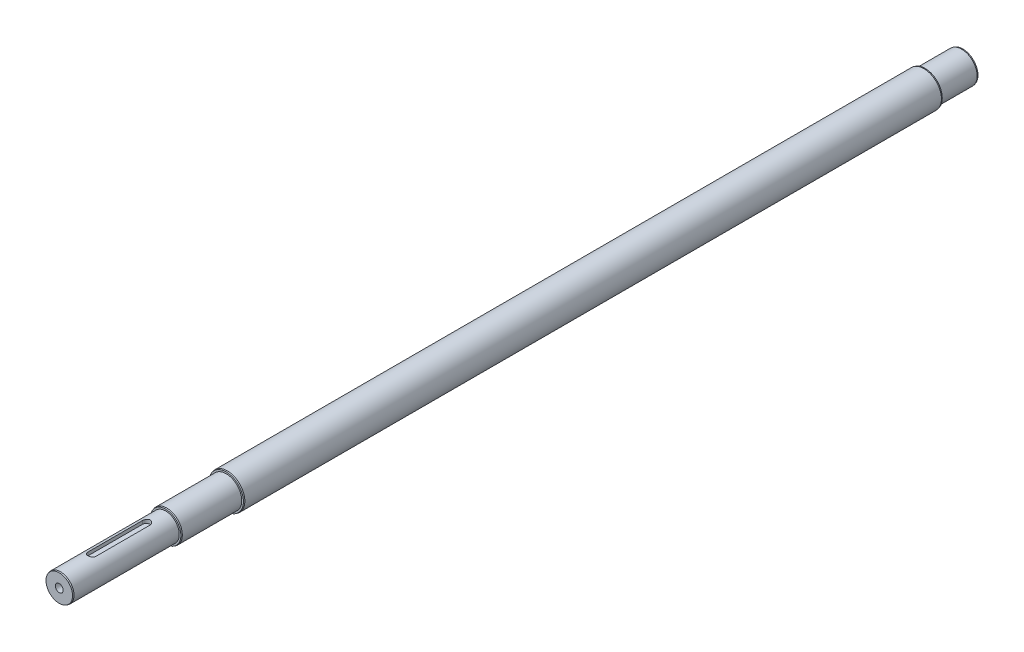
SolidWorks part; units mm, degrees
ref_plane "前视基准面" through (0, 0, 0) normal (0, 0, 1) x (1, 0, 0)
ref_plane "上视基准面" through (0, 0, 0) normal (0, 1, 0) x (1, 0, 0)
ref_plane "右视基准面" through (0, 0, 0) normal (1, 0, 0) x (0, 0, -1)
sketch "草图1" plane through (0, 0, 0) normal (0, 0, 1) x (1, 0, 0)
  circle A0 centre (0, 0) radius 22.5
  dimension "D1" = 45
extrude "凸台-拉伸1" add sketch "草图1" along normal blind 900 contours A0
sketch "草图2" plane through (0, 0, 900) normal (0, 0, 1) x (1, 0, 0)
  circle A0 centre (0, 0) radius 20
  dimension "D1" = 40
extrude "凸台-拉伸2" add sketch "草图2" along normal blind 78
sketch "草图3" plane through (0, 0, 978) normal (0, 0, 1) x (1, 0, 0)
  circle A0 centre (0, 0) radius 17.5
  dimension "D1" = 35
extrude "凸台-拉伸3" add sketch "草图3" along normal blind 137
sketch "草图4" plane through (0, 0, 0) normal (0, 0, -1) x (-1, 0, 0)
  circle A0 centre (0, 0) radius 20
  dimension "D1" = 40
extrude "凸台-拉伸4" add sketch "草图4" along normal blind 48.5
chamfer "倒角1" distance 1.5 angle 15 4 edges at (22.5, 0, 900) (-20, 0, -48.5) (17.5, 0, 1115) (20, 0, 978)
ref_plane "基准面1" through (0, 17.5, 0) normal (0, 1, 0) x (1, 0, 0)
sketch "草图5" plane through (0, 17.5, 0) normal (0, 1, 0) x (1, 0, 0)
  line L0 (0, -1003) -> (0, -1073) construction
  line L1 (5, -1003) -> (5, -1073)
  line L2 (-5, -1003) -> (-5, -1073)
  line L3 (0, -978) -> (0, -934.3002)
  line L4 (-17.5, -978) -> (17.5, -978) construction
  arc A0 (5, -1003) -> (-5, -1003) centre (0, -1003) ccw
  arc A1 (-5, -1073) -> (5, -1073) centre (0, -1073) ccw
  point P2 (0, -1038)
  dimension "D1" = 10
  dimension "D3" = 25
  dimension "D2" = 70
extrude "切除-拉伸1" cut sketch "草图5" against normal blind 5 contours L1 A1 L2 A0
sketch "草图6" plane through (0, 0, 1115) normal (0, 0, 1) x (1, 0, 0)
  circle A0 centre (0, 0) radius 6
  dimension "D1" = 12
hole_wizard "M12 螺纹孔1" positions "草图7" profile "草图8" tap size "M12" standard "GB"
sketch "草图7" plane through (0, 0, 1115) normal (0, 0, 1) x (1, 0, 0)
  point P0 (0, 0)
sketch "草图8" plane through (0, 0, 1115) normal (1, 0, 0) x (0, -1, 0)
  line L0 (0, 0) -> (0, 32.3144)
  line L1 (0, 32.3144) -> (5.1, 29.25)
  line L2 (5.1, 29.25) -> (5.1, 0)
  line L5 (5.1, 0) -> (0, 0)
  line L10 (0, 32.3144) -> (-5.1, 29.25) construction
  line L11 (0, -6.35) -> (0, 107.95) construction
  dimension "螺纹孔钻头直径" = 10.2
  dimension "螺纹孔钻头深度" = 29.25
  dimension "导头角度" = 118
cosmetic thread "孔螺蚊线1" parameters "D1"=24, "D2"=12
sketch "草图9" plane through (0, 0, -48.5) normal (0, 0, -1) x (-1, 0, 0)
  circle A0 centre (0, 0) radius 6
  dimension "D1" = 12
hole_wizard "M10 螺纹孔1" positions "草图10" profile "草图11" tap size "M10" standard "IS"
sketch "草图10" plane through (0, 0, -48.5) normal (0, 0, -1) x (-1, 0, 0)
  point P0 (0, 0)
sketch "草图11" plane through (0, 0, -48.5) normal (1, 0, 0) x (0, 1, 0)
  line L0 (0, 0) -> (0, 27.0537)
  line L1 (0, 27.0537) -> (4.25, 24.5)
  line L2 (4.25, 24.5) -> (4.25, 0)
  line L5 (4.25, 0) -> (0, 0)
  line L10 (0, 27.0537) -> (-4.25, 24.5) construction
  line L11 (0, -6.35) -> (0, 107.95) construction
  dimension "螺纹孔钻头直径" = 8.5
  dimension "螺纹孔钻头深度" = 24.5
  dimension "导头角度" = 118
cosmetic thread "孔螺蚊线2" parameters "D1"=20, "D2"=10
chamfer "倒角2" distance 1.5 angle 15 1 edges at (22.5, 0, 0)
fillet "圆角1" radius 1 1 edges at (-20, 0, 0)
